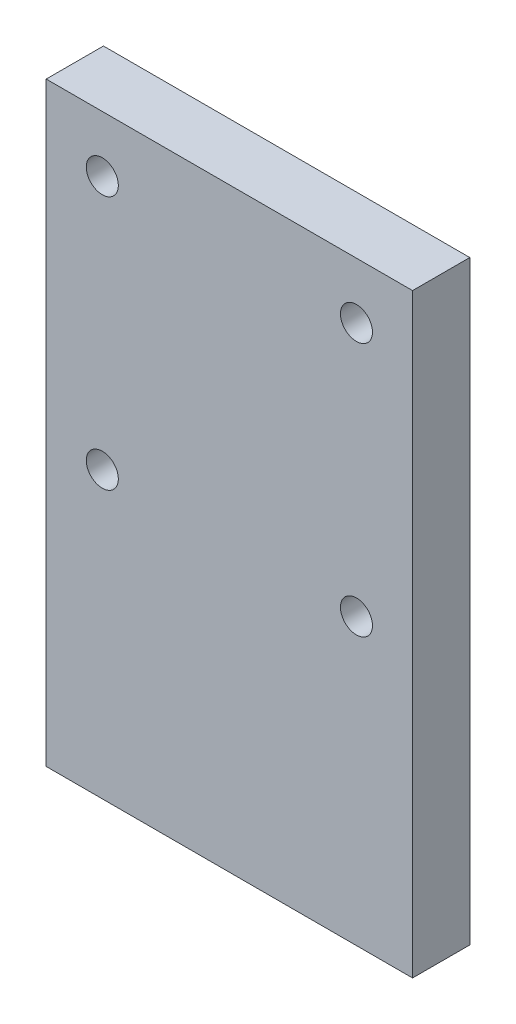
SolidWorks part; units mm, degrees
material "XRAAT"
ref_plane "前视基准面" through (0, 0, 0) normal (0, 0, 1) x (1, 0, 0)
ref_plane "上视基准面" through (0, 0, 0) normal (0, 1, 0) x (1, 0, 0)
ref_plane "右视基准面" through (0, 0, 0) normal (1, 0, 0) x (0, 0, -1)
sketch "草图1" plane through (0, 0, 0) normal (0, 0, 1) x (1, 0, 0)
  line L1 (80, -130) -> (-80, -130)
  line L2 (80, -130) -> (80, 130)
  line L3 (80, 130) -> (-80, 130)
  line L4 (-80, -130) -> (-80, 130)
  line L5 (80, -130) -> (-80, 130) construction
  line L6 (80, 130) -> (-80, -130) construction
  point P0 (0, 0)
  dimension "D1" = 260
  dimension "D2" = 160
extrude "凸台-拉伸1" add sketch "草图1" along normal blind 25
hole_wizard "M16 螺纹孔1" positions "草图2" profile "草图3" tap size "M16" standard "GB" end condition up to next
sketch "草图2" plane through (0, 0, 25) normal (0, 0, 1) x (1, 0, 0)
  line L0 (0, 0) -> (0, 130) construction
  line L1 (80, 130) -> (-80, 130) construction
  point P0 (-55.5, 105.5)
  point P2 (-55.5, -5.5)
  point P11 (55.5, -5.5)
  point P12 (55.5, 105.5)
  dimension "D1" = 111
  dimension "D2" = 24.5
  dimension "D3" = 111
sketch "草图3" plane through (-55.5, 105.5, 25) normal (1, 0, 0) x (0, -1, 0)
  line L0 (0, 0) -> (0, 25)
  line L1 (0, 25) -> (7, 25)
  line L2 (7, 25) -> (7, 0)
  line L5 (7, 0) -> (0, 0)
  line L11 (0, -6.35) -> (0, 107.95) construction
  dimension "通孔螺纹孔钻头直径" = 14
  dimension "通孔螺纹孔钻头深度" = 25
cosmetic thread "孔螺蚊线1" parameters "D2"=16
cosmetic thread "孔螺蚊线2" parameters "D2"=16
cosmetic thread "孔螺蚊线3" parameters "D2"=16
cosmetic thread "孔螺蚊线4" parameters "D2"=16
